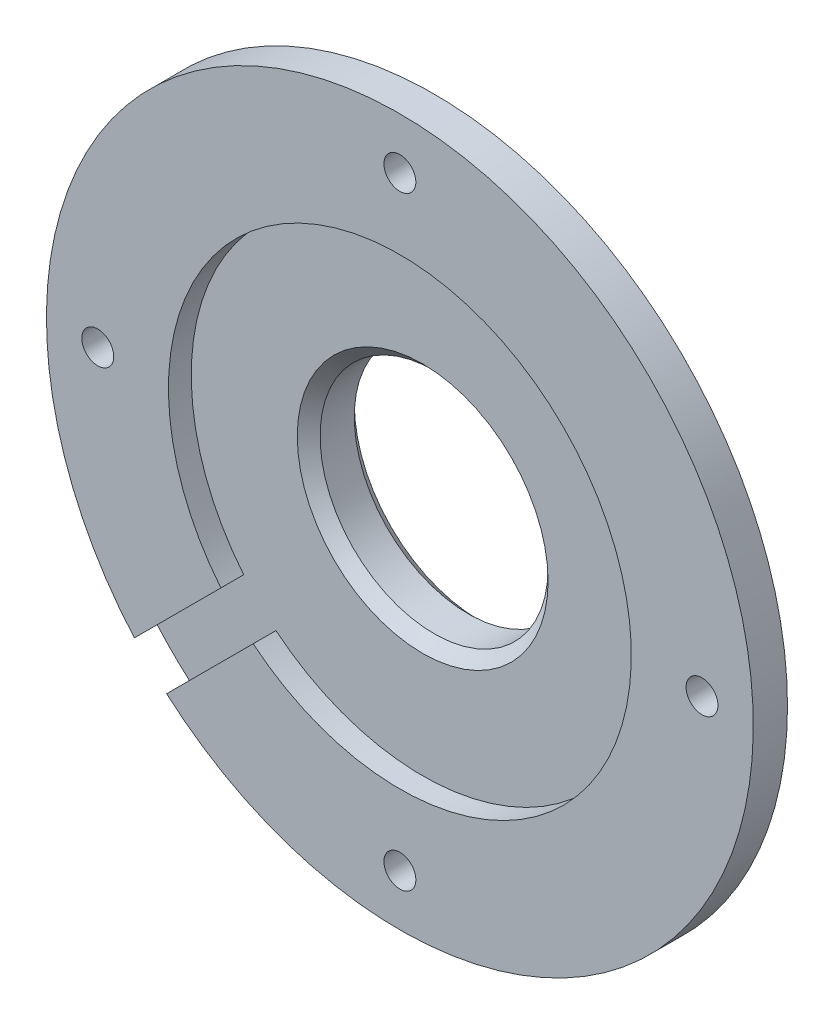
SolidWorks part; units mm, degrees
ref_plane "Front Plane" through (0, 0, 0) normal (0, 0, 1) x (1, 0, 0)
ref_plane "Top Plane" through (0, 0, 0) normal (0, 1, 0) x (1, 0, 0)
ref_plane "Right Plane" through (0, 0, 0) normal (1, 0, 0) x (0, 0, -1)
other "Configuration Table"
sketch "Sketch1" plane through (0, 0, 0) normal (0, 0, 1) x (1, 0, 0)
  circle A0 centre (0, 0) radius 12
  dimension "D1" = 24
extrude "Boss-Extrude1" add sketch "Sketch1" along normal blind 2
sketch "Sketch2" plane through (0, 0, 2) normal (0, 0, 1) x (1, 0, 0)
  circle A0 centre (0, 0) radius 15.5
  circle A1 centre (0, 0) radius 13.25 construction
  circle A2 centre (0, 13.25) radius 0.7
  circle A3 centre (13.25, 0) radius 0.7
  circle A4 centre (0, -13.25) radius 0.7
  circle A5 centre (-13.25, 0) radius 0.7
  point P15 (0, 0)
  dimension "D1" = 31
  dimension "D2" = 26.5
  dimension "D3" = 1.4
  dimension "D4" = 4
extrude "Boss-Extrude2" add sketch "Sketch2" along normal blind 1.5
sketch "Sketch3" plane through (0, 0, 3.5) normal (0, 0, 1) x (1, 0, 0)
  circle A0 centre (0, 0) radius 10.15
  dimension "D1" = 20.3
extrude "Cut-Extrude1" cut sketch "Sketch3" against normal blind 1
fillet "Fillet1" radius 1.2 1 edges at (12, 0, 0)
sketch "Sketch4" plane through (0, 0, 2) normal (0, 0, -1) x (-1, 0, 0)
  circle A0 centre (0, 13.25) radius 1.25
  circle A1 centre (13.25, 0) radius 1.25
  circle A2 centre (0, -13.25) radius 1.25
  circle A3 centre (-13.25, 0) radius 1.25
  point P12 (0, 0)
  dimension "D1" = 2.5
  dimension "D2" = 4
extrude "Cut-Extrude2" cut sketch "Sketch4" against normal blind 0.5
sketch "Sketch5" plane through (0, 0, 0) normal (0, 0, -1) x (-1, 0, 0)
  circle A0 centre (0, 0) radius 5
  dimension "D1" = 10
extrude "Cut-Extrude3" cut sketch "Sketch5" against normal through all
chamfer "Chamfer1" distance 0.5 angle 45 2 edges at (-5, 0, 0) (5, 0, 2.5)
sketch "Sketch6" plane through (0, 0, 3.5) normal (0, 0, 1) x (1, 0, 0)
  line L0 (0, 0) -> (0, 13.25) construction
  line L5 (-0.7071, 0.7071) -> (0.7071, -0.7071)
  line L6 (0, 0) -> (-10.9602, -10.9602) construction
  line L7 (-11.6673, -10.253) -> (-10.253, -11.6673)
  line L8 (0.7071, -0.7071) -> (-10.253, -11.6673)
  line L9 (-0.7071, 0.7071) -> (-11.6673, -10.253)
  dimension "D1" = 135
  dimension "D2" = 2
extrude "Cut-Extrude4" cut sketch "Sketch6" against normal blind 1
